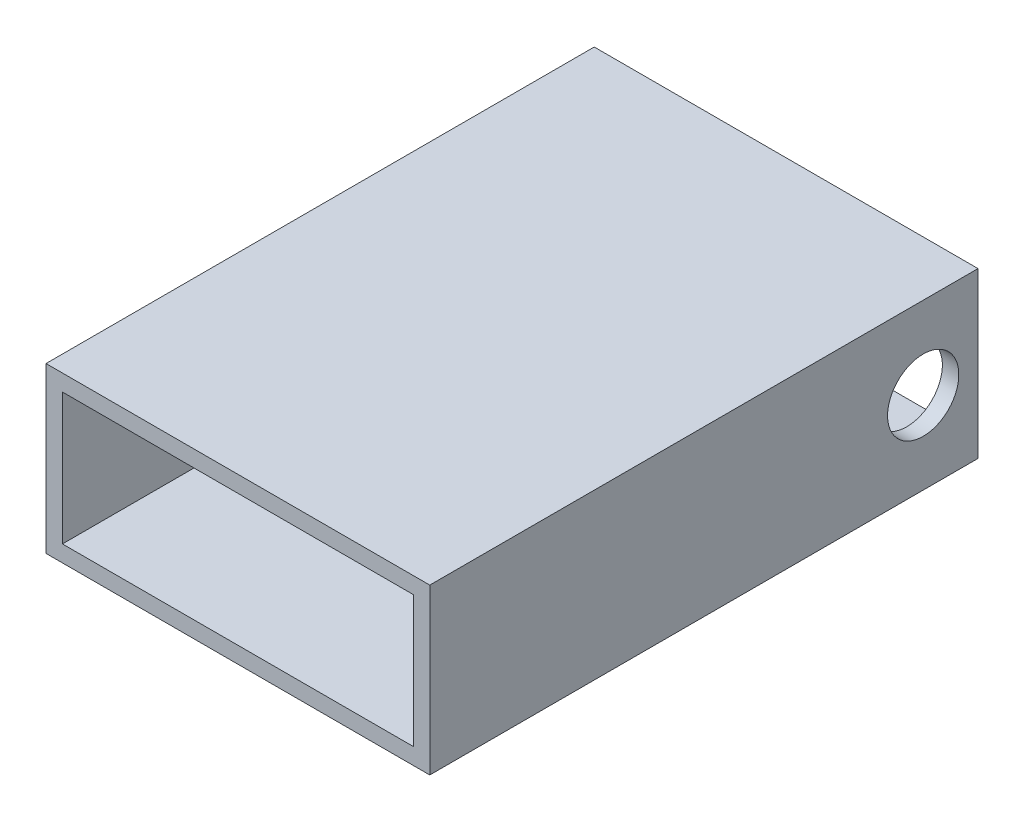
SolidWorks part; units mm, degrees
ref_plane "前视基准面" through (0, 0, 0) normal (0, 0, 1) x (1, 0, 0)
ref_plane "上视基准面" through (0, 0, 0) normal (0, 1, 0) x (1, 0, 0)
ref_plane "右视基准面" through (0, 0, 0) normal (1, 0, 0) x (0, 0, -1)
sketch "草图1" plane through (0, 0, 0) normal (0, 0, 1) x (1, 0, 0)
  line L0 (0, 0) -> (0, 30)
  line L1 (0, 30) -> (70, 30)
  line L2 (70, 30) -> (70, 0)
  line L3 (70, 0) -> (0, 0)
extrude "凸台-拉伸1" add sketch "草图1" along normal blind 100
sketch "草图2" plane through (0, 0, 0) normal (-1, 0, 0) x (0, 0, 1)
  line L0 (0, 15) -> (10, 15)
  line L2 (0, 30) -> (0, 0) construction
  circle A0 centre (10, 15) radius 6.5
shell "抽壳1" thickness 3
extrude "切除-拉伸2" cut sketch "草图2" against normal blind 100
